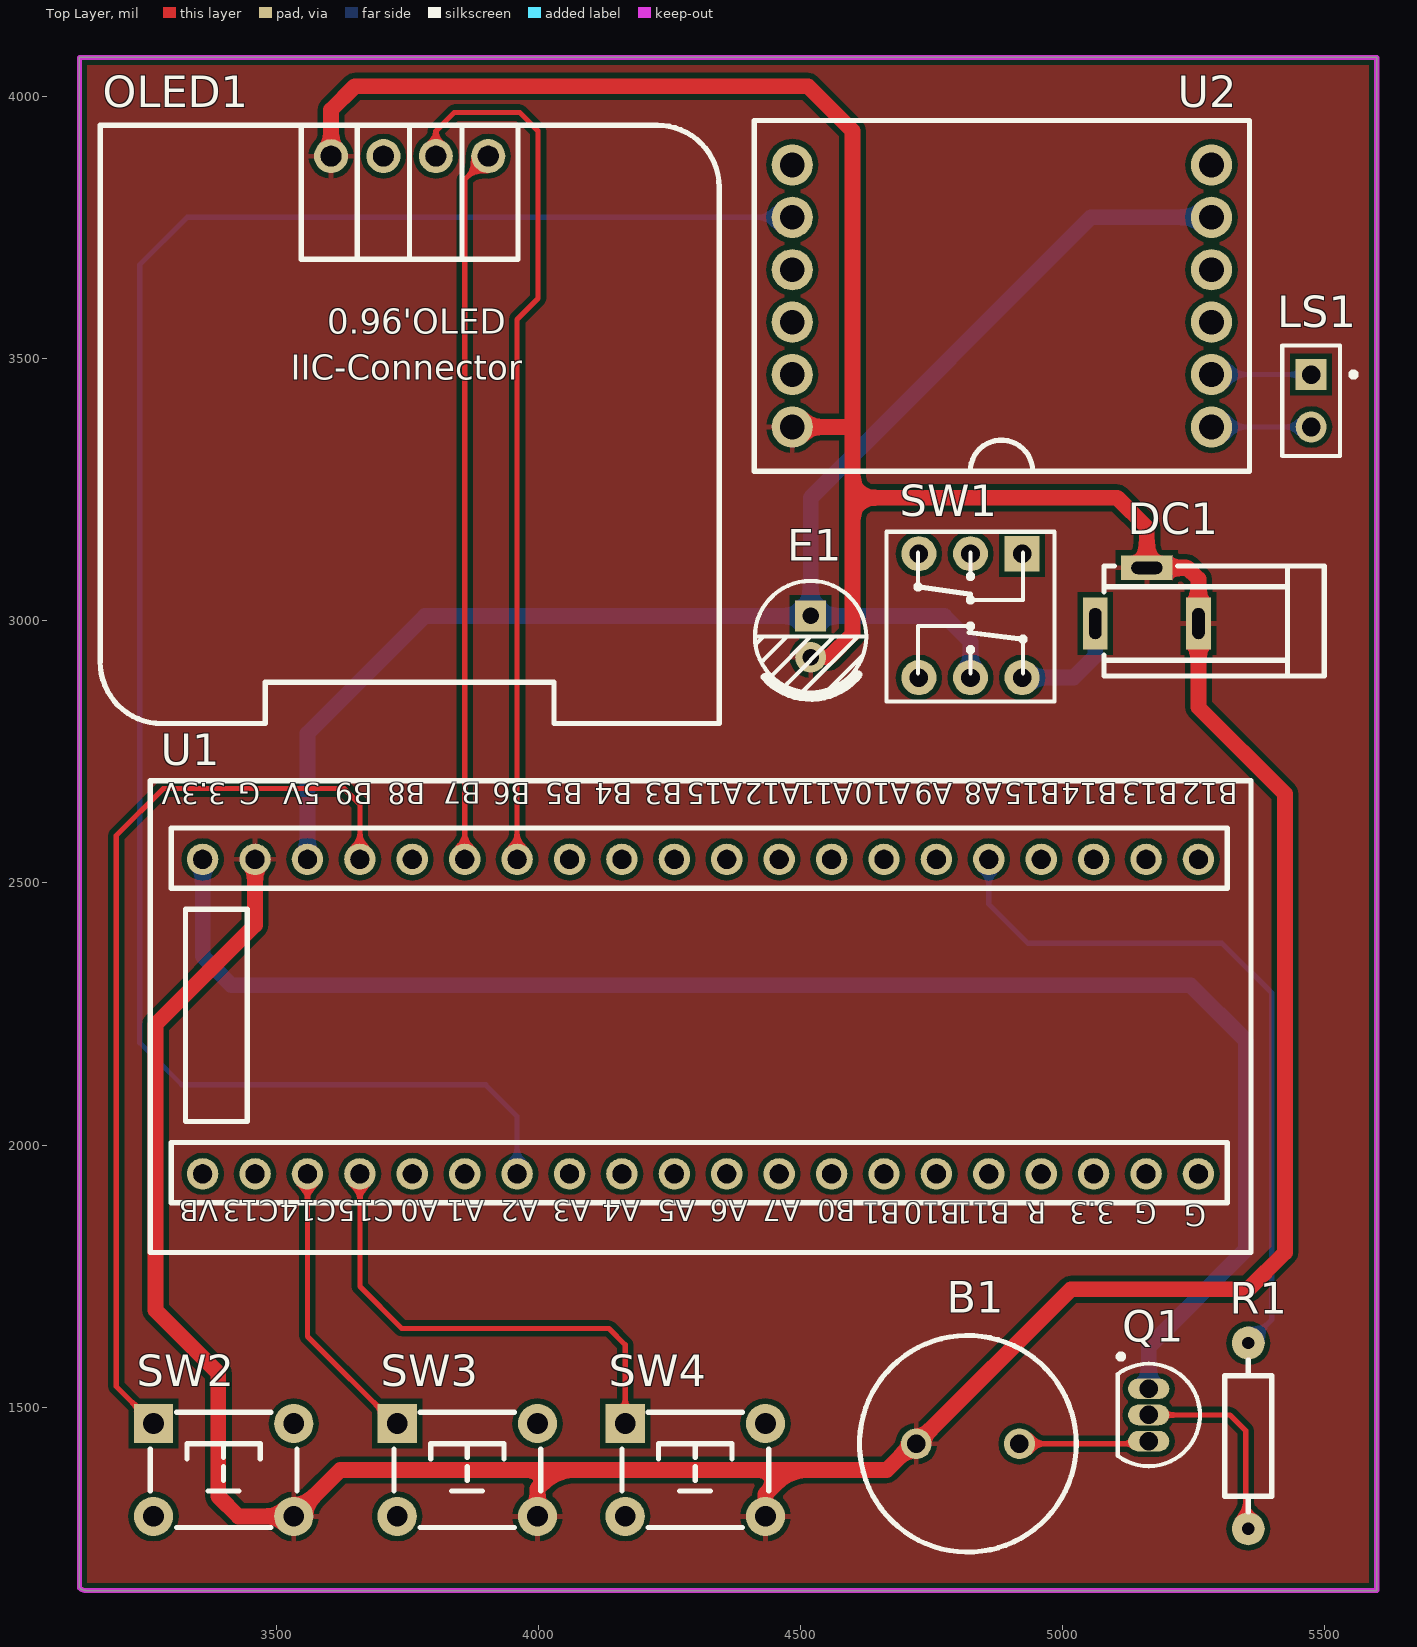
[diagram p0: Top Layer view]
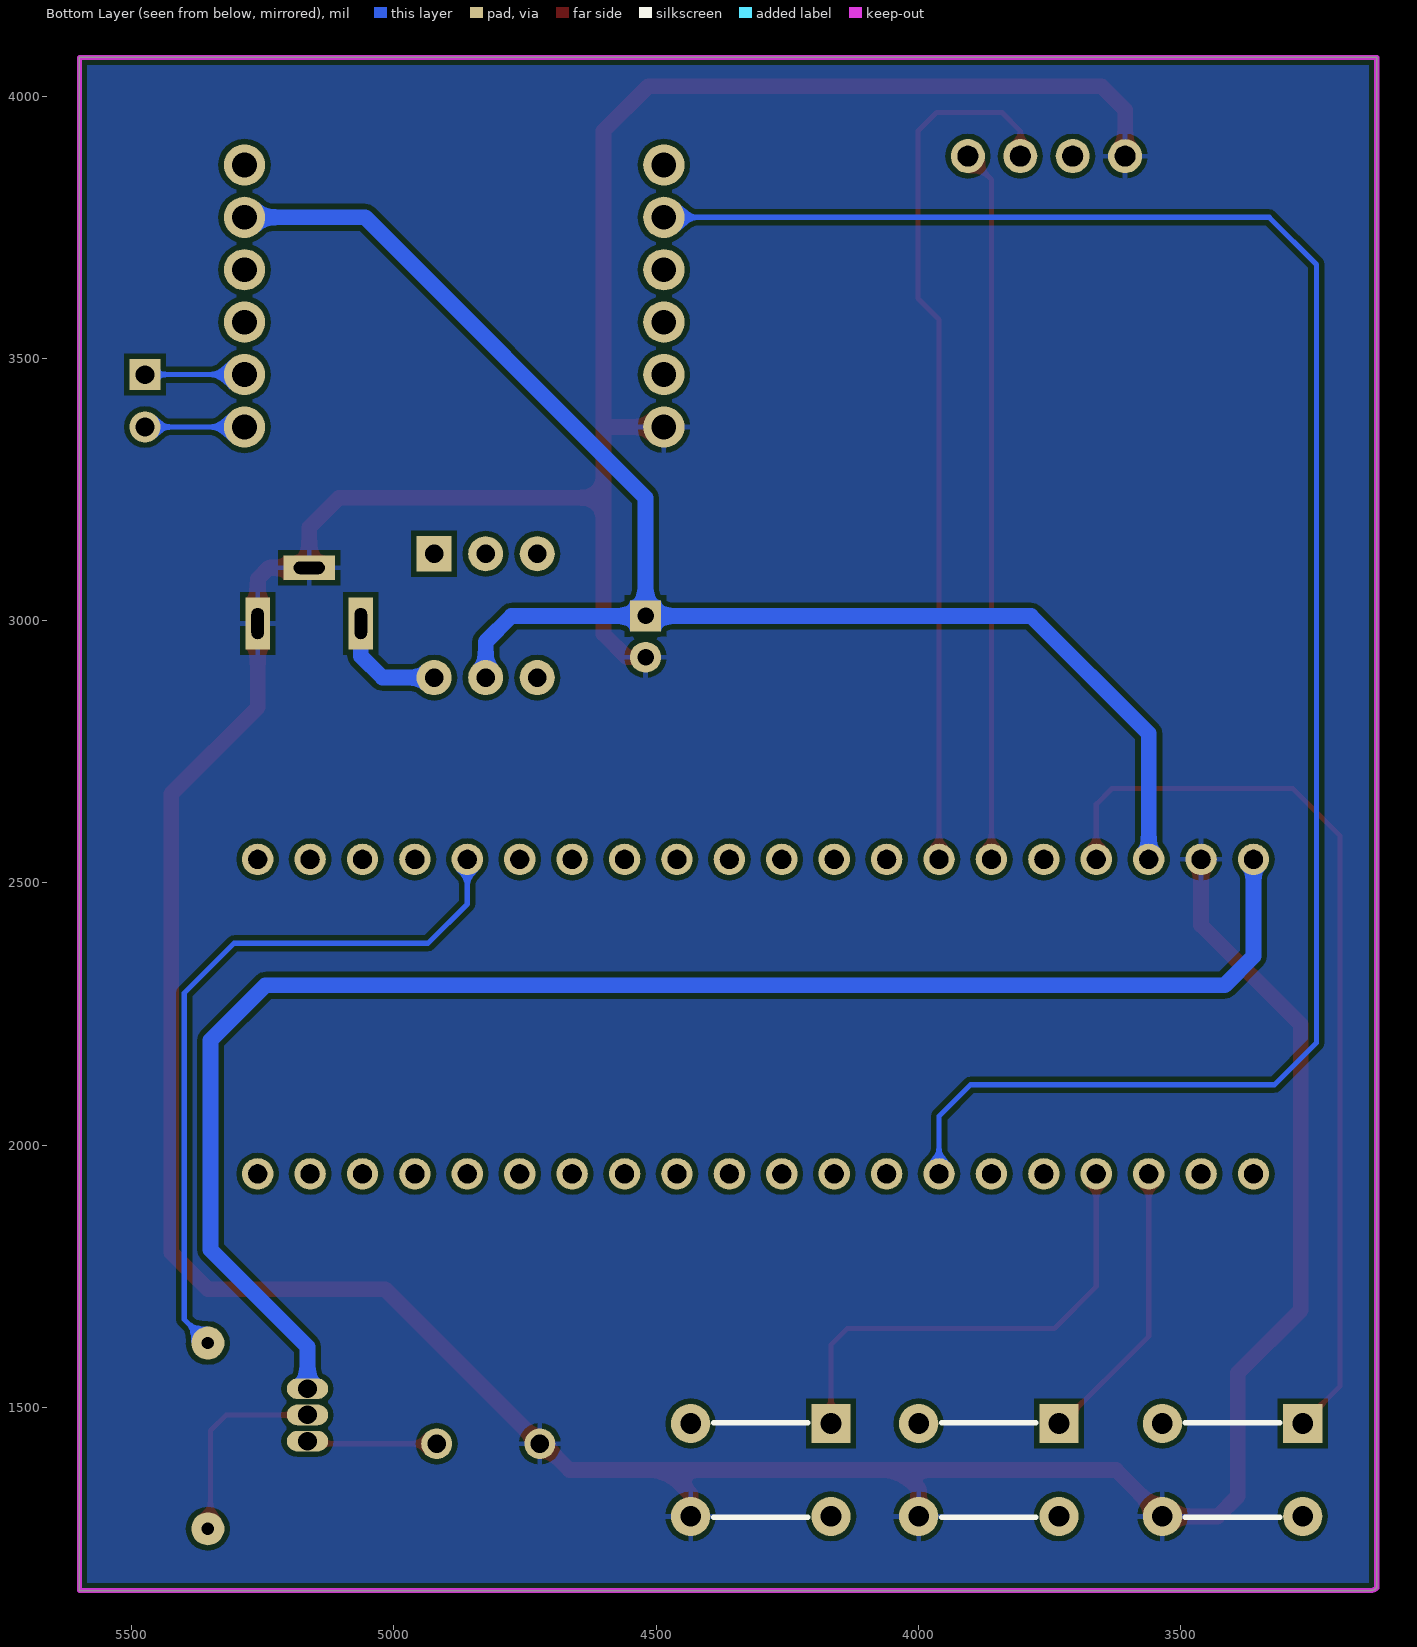
[diagram p1: Bottom Layer view, seen from below]
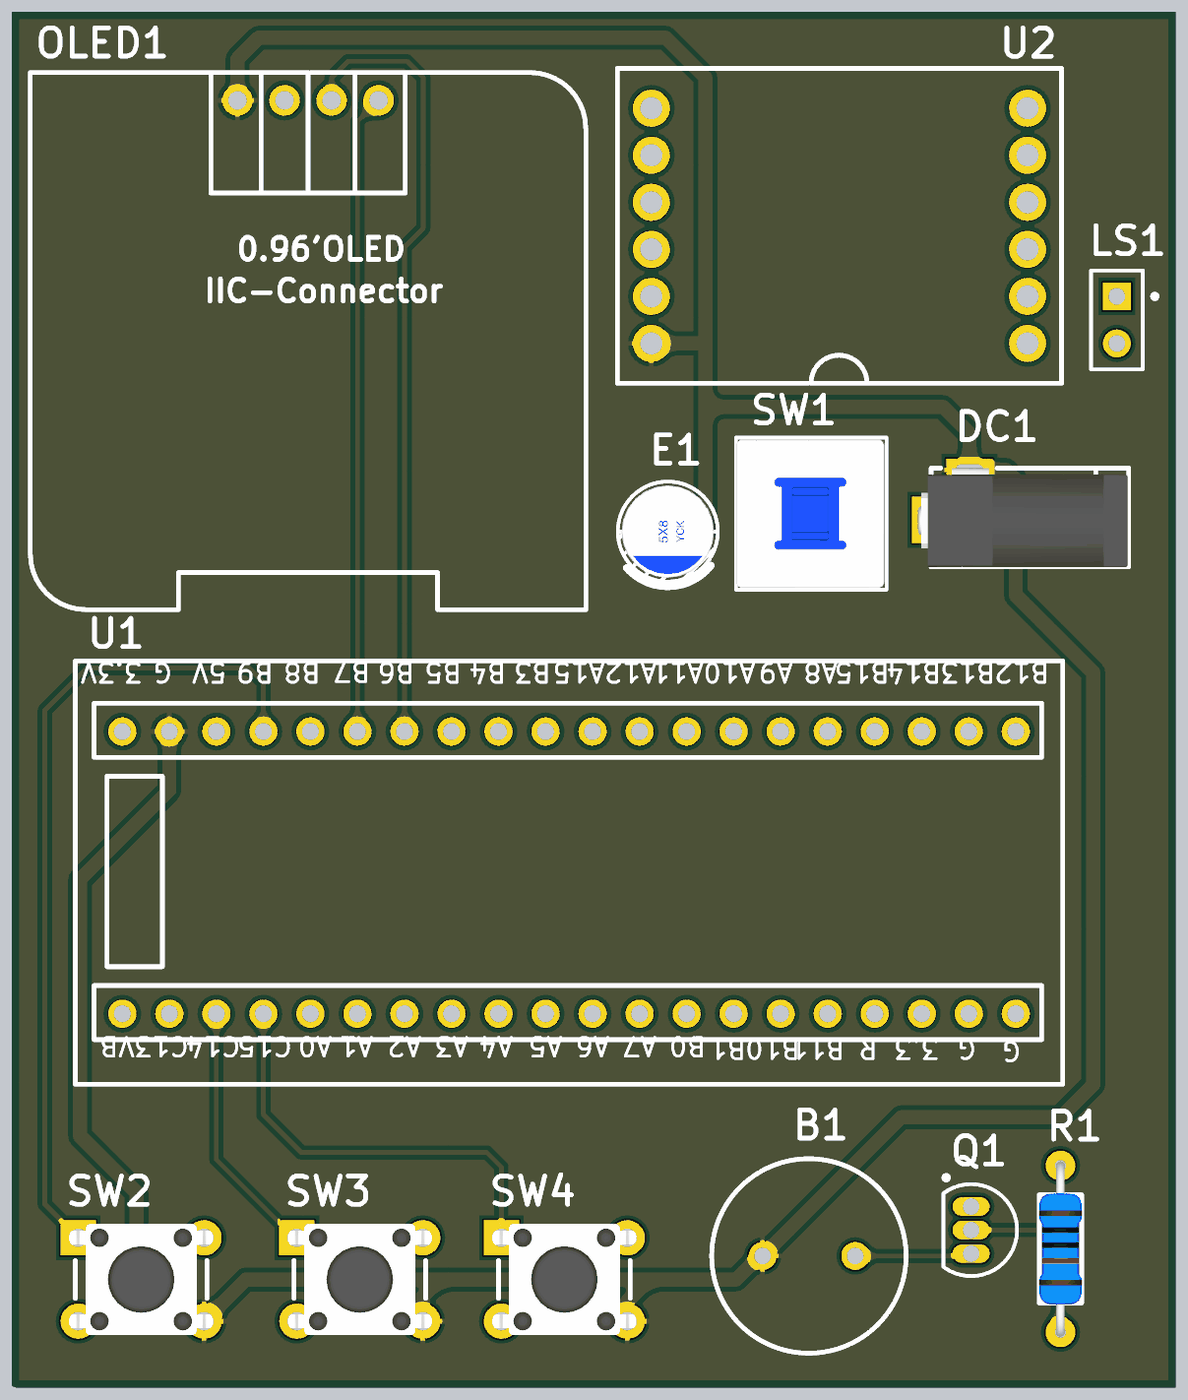
[diagram p2: 3D render of the assembled board from above, using the file's embedded part models]
# Altium PCB MISC82785.PcbDoc
Units mil, origin at the board's own origin, x right, y up, seen from the top; angles counter-clockwise.
Board outline 2475 x 2925 mil, 2 copper layers (Top Layer, Bottom Layer); 13 components, 16 nets, 88 pads, 0 vias.

## Layer stack, top to bottom (the 12.6 mil dielectric is the usual default, probably not edited)
Top Solder: solder mask 0.4, Solder Resist, Dk 3.5
Top Layer: signal copper 1.4
Dielectric 1: dielectric 12.6, FR-4, Dk 4.8
Bottom Layer: signal copper 1.4
Bottom Solder: solder mask 0.4, Solder Resist, Dk 3.5

## Board outline
3125,1155 ccw(c3137.07,1167.07) 3137.07,1150 5600,1150 5600,4075 3125,4075

## Design rules (kind name [scope] priority, off if disabled: settings)
Clearance [All] p1: gap=10
MinimumSolderMaskSliver [All] p1: minsoldermaskwidth=0
PolygonConnect [All] p1: connectstyle=Relief reliefconductorwidth=10 reliefentries=4 polygonreliefangle="90 Angle" airgapwidth=10
RoutingVias [All] p1: holewidth=28 width=50 viastyle="Through Hole" minholewidth=28 minwidth=50 maxholewidth=28 maxwidth=50
ShortCircuit [All] p1: allowed=TRUE
SilkToSilkClearance [All] p1: silktosilkclearance=0
SilkToSolderMaskClearance [IsPad] p1: minsilkscreentomaskgap=0 clearancetoexposedcopper=TRUE
SolderMaskExpansion [All] p1: expansion=4
Width [All] p1: maxlimit=30 minlimit=10 preferedwidth=10
26 further rules are at their usual default settings.

## Components (designator, comment, footprint, x,y, rotation, side; value= is the part's Value field where it differs from the comment)
B1 "Motor" RB5-10.5 4820,1430 r180 top
DC1 "DC_Socket" DC-002 5063.15,2995 r0 top
E1 "470uF" "CS 2.0*5*8 - C" 4520,2970 r90 top
LS1 "Speaker" PIN2 5475,3470 r270 top
OLED1 "0.96OLED_4P_MODULE_JX" 0.96OLED_4P 3755,3375 r0 top
Q1 "9012" TO-92A 5165,1485 r180 top
R1 "1K" "RS 1/4W" 5355,1445 r270 top
SW1 "KET 8X8" "KFT DIP-8X8" 4825,3010 r180 top
SW2 "6x6x5" "TSW DIP-6*6*6" 3400,1380 r0 top
SW3 "6x6x5" "TSW DIP-6*6*6" 3865,1380 r0 top
SW4 "6x6x5" "TSW DIP-6*6*6" 4300,1380 r0 top
U1 "STM32F103C8T6 minimum system board" STM32核心板 4086,3446.5 r90 top
U2 "MY1680U-12P_1" COMM-TH_MY1680-12P 4885,3620 r0 top

## Footprints (in the part's own frame and the unit in brackets; to place one, negate y for a bottom-side part, rotate by r counter-clockwise, add the part's x,y. Pads: shape width x height; smd on the part's side, far side on the other; paste and mask are expansions set on the pad)
0.96OLED_4P [mm]
  round 1.65 hole 1 slot 1.005 at 0 deg paste+0 mask+0.051: 1(-3.811,12.997) 2(-1.271,13) 3(1.269,13) 4(3.809,13)
  silkscreen extent -15,-14.5 15,14.5
COMM-TH_MY1680-12P [mm]
  round 2 hole 1.2 paste+0 mask+0.05: 1(10.16,-6.35) 2(10.16,-3.81) 3(10.16,-1.27) 4(10.16,1.27) 5(10.16,3.81) 6(10.16,6.35) 7(-10.16,6.35) 8(-10.16,3.81) 9(-10.16,1.27) 10(-10.16,-1.27) 11(-10.16,-3.81) 12(-10.16,-6.35)
  silkscreen extent -12,-8.5 12,8.5
"CS 2.0*5*8 - C" [mm] "脚距2mm , 直径5mm , 高8mm"
  rect 1.5x1.5 hole 0.8: 1(1,0)
  round 1.5 hole 0.8: 2(-1,0)
  silkscreen extent -2.96,-2.7 2.7,2.7, body extent -2.5,-2.5 2.5,2.5, height 8.02
DC-002 [mm] "3.5X1.1mm"
  rect 1.2x2.5 hole 0.6 slot 1.5 at 90 deg: 1(0,0) 2(5,0)
  rect 2.5x1.2 hole 0.6 slot 1.5 at 0 deg: 3(2.5,2.7)
  silkscreen extent 0.43,-2.54 11.1,2.79, body extent -0.25,-2.55 11.05,2.8, height 7.3
"KFT DIP-8X8" [mm] "自锁开关，规格：8*8mm"
  rect 1.7x1.7 hole 0.9: 1(-2.5,-3)
  round 1.7 hole 0.9: 2(0,-3) 3(2.5,-3) 4(2.5,3) 5(0,3) 6(-2.5,3)
  silkscreen extent -4.06,-4.06 4.06,4.15, body extent -3.95,-3.95 4.05,4.05, height 13.1
PIN2 [mm] "Photosensitive Diode; 2 Leads"
  rect 1.5x1.5 hole 0.9: 1(0,0)
  round 1.5 hole 0.9: 2(2.54,0)
  silkscreen extent -1.4,-1.4 3.94,2.18
RB5-10.5 [mm] "Capacitor (Radial); 2 Leads"
  round 1.5 hole 0.9: 1(-2.5,0) 2(2.5,0)
  silkscreen extent -5.25,-5.25 5.25,5.25
"RS 1/4W" [mm] "直插色环电阻，脚距9mm，直径2.3mm"
  round 1.6 hole 0.6: 1(-4.5,0) 2(4.5,0)
  silkscreen extent -3.68,-1.14 3.68,1.14, body extent -4.72,-1.16 4.73,1.16, height 2.32
STM32核心板 [mil]
  round 60 hole 36 slot 36.2 at 0 deg paste+0 mask+2: 1(-1501.5,726) 2(-1501.5,626) 3(-1501.5,526) 4(-1501.5,426) 5(-1501.5,326) 6(-1501.5,226) 7(-1501.5,126) 8(-1501.5,26) 9(-1501.5,-74) 10(-1501.5,-174) 11(-1501.5,-274) 12(-1501.5,-374) 13(-1501.5,-474) 14(-1501.5,-574) 15(-1501.5,-674) 16(-1501.5,-774) 17(-1501.5,-874) 18(-1501.5,-974) 19(-1501.5,-1074) 20(-1501.5,-1174) 21(-901.5,-1174) 22(-901.5,-1074) 23(-901.5,-974) 24(-901.5,-874) 25(-901.5,-774) 26(-901.5,-674) 27(-901.5,-574) 28(-901.5,-474) 29(-901.5,-374) 30(-901.5,-274) 31(-901.5,-174) 32(-901.5,-74) 33(-901.5,26) 34(-901.5,126) 35(-901.5,226) 36(-901.5,326) 37(-901.5,426) 38(-901.5,526) 39(-901.5,626) 40(-901.5,726)
  silkscreen extent -1652,-1274 -751,826
TO-92A [mm] "TO, Flat Index; 3 In-Line, Axial Leads; Body Dia. 4.5mm; Leads 0.51 x 0.48 mm (max)"
  oval 2x1 hole 0.9: 1(0,-1.27) 2(0,0) 3(0,1.27)
  silkscreen extent -2.48,-2.95 1.5,2.48, body extent -2.48,-2.5 1.5,2.5, height 6.86
"TSW DIP-6*6*6" [mm] "6*6*6mm"
  rect 1.9x1.9 hole 1: 1(-3.4,2.25)
  round 1.9 hole 1: 2(-3.4,-2.25) 3(3.4,-2.25) 4(3.4,2.25)
  silkscreen extent -3.56,-2.79 3.56,2.79, body extent -4.11,-3 4.11,3, height 5.95

## Part data
B1: "Motor, General Kind"
E1: library part CS, "THT solid capacitor"
LS1: "Loudspeaker"
Q1: library part 2N3906, "PNP General Purpose Amplifier"
R1: library part R-S, "Color-band resistor"
SW1: "8*8 self-locking switch"
SW2 SW3 SW4: library part "TSW DIP-6x6", "THT 6x6 tactile switch"
U1: library part STM32F103C8T6最小系统板

## Nets (pads, with @x,y where several pads share a name; then routed paths per layer and width w, separated by ;. In a path a pad name is that pad's centre, name@x,y a point inside that pad or via, vN(x,y) a via of type N, cw(c..) or ccw(c..) an arc to the next point about the centre after c; other vN are vias at no path point)
3.3V: Q1.1 U1.40 | length 2982.9
  Bottom Layer w30: U1.40 3360,2360 3415,2305 5245,2305 5350,2200 5350,1800 5165,1615 Q1.1
+5: E1.1 SW1.5 U1.38 U2.5 | length 2898.7
  Bottom Layer w30: U1.38 3560,2785 3784.37,3009.37 E1.1 ; SW1.5 4825,2960 4775.63,3009.37 E1.1 ; U2.5 5055,3770 4520,3235 E1.1
GND: B1.2 DC1.2 DC1.3 E1.2 OLED1.1 SW2.3 SW3.3 SW4.3 U1.39 U2.12 | length 8251.6
  Top Layer w30: U1.39 3460,2420 3270,2230 3270,1685 3390,1565 3390,1330 3428.58,1291.42 SW2.3 3622.44,1380 4035,1380 ; OLED1.1 3604.95,3974.95 3650,4020 4515,4020 4600,3935 4600,3380 ; SW3.3 3998.86,1343.86 4035,1380 ; SW4.3 4433.86,1333.86 4480,1380 ; U2.12 4590,3370 4600,3380 ; E1.2 4555.63,2930.63 4600,2975 4600,3235 ; 4035,1380 4480,1380 ; 4480,1380 4665,1380 4715,1430 B1.2 5016.57,1725 5355,1725 5425,1795 5425,2670 5260,2835 DC1.2 5260,3080 5238.7,3101.3 DC1.3 5161.57,3178.43 5105,3235 4600,3235 ; 4600,3235 4600,3380
NetB1_1: B1.1 Q1.3 | length 248.6
  Top Layer w10: B1.1 5160,1430 Q1.3
NetDC1_1: DC1.1 SW1.6 | length 218.7
  Bottom Layer w30: SW1.6 5021.89,2891.89 5063.15,2933.15 DC1.1
NetLS1_1: LS1.1 U2.2 | length 190
  Bottom Layer w10: U2.2 LS1.1
NetLS1_2: LS1.2 U2.1 | length 190
  Bottom Layer w10: U2.1 LS1.2
NetQ1_2: Q1.2 R1.2 | length 386.7
  Top Layer w10: Q1.2 5320,1485 5350,1455 5350,1272.83 R1.2
PA2: U1.7 U2.8 | length 3655.3
  Bottom Layer w10: U1.7 3960,2055 3900,2115 3320,2115 3240,2195 3240,3680 3330,3770 U2.8
PA8: R1.1 U1.25 | length 1381.9
  Bottom Layer w10: U1.25 4860,2460 4935,2385 5305,2385 5400,2290 5400,1667.17 R1.1
PB6: OLED1.3 U1.34 | length 1678.8
  Top Layer w10: OLED1.3 3804.95,3934.95 3840,3970 3965,3970 4000,3935 4000,3615 3960,3575 U1.34
PB7: OLED1.4 U1.35 | length 1360.4
  Top Layer w10: U1.35 3860,3841.86 OLED1.4
PB9: SW2.1 U1.37 | length 1770.6
  Top Layer w10: SW2.1 3195,1539.72 3195,2590 3285,2680 3630,2680 3660,2650 U1.37
PC14: SW3.1 U1.3 | length 550.1
  Top Layer w10: U1.3 3560,1635 3726.42,1468.58 SW3.1
PC15: SW4.1 U1.4 | length 917.5
  Top Layer w10: U1.4 3660,1730 3740,1650 4135,1650 4166.14,1618.86 SW4.1
VCC: OLED1.2
pads on no net: SW1.1 SW1.2 SW1.3 SW1.4 SW2.2 SW2.4 SW3.2 SW3.4 SW4.2 SW4.4 U1.1 U1.2 U1.5 U1.6 U1.8 U1.9 U1.10 U1.11 U1.12 U1.13 U1.14 U1.15 U1.16 U1.17 U1.18 U1.19 U1.20 U1.21 U1.22 U1.23 U1.24 U1.26 U1.27 U1.28 U1.29 U1.30 U1.31 U1.32 U1.33 U1.36 U2.3 U2.4 U2.6 U2.7 U2.9 U2.10 U2.11

## Polygon pours and split planes (outlines as drawn)
GND on Bottom Layer "D" (solid, remove dead copper, pour order 0): 2520,4225 2600,4305 5725,4305 5725,1040 5755,1010 5700,955 2755,955
GND on Top Layer "D" (solid, remove dead copper, pour order 2): 2990,4180 5655,4180 5695,4220 5710,4205 5710,1000 2960,1000 2915,1045

## Keep-outs
Keep-Out Layer:
  lines w10: 3125,1155 ccw(c3137.07,1167.07) 3137.07,1150 3210,1150 5600,1150 5600,3995 5600,4075 3170,4075 3125,4075 3125,1155